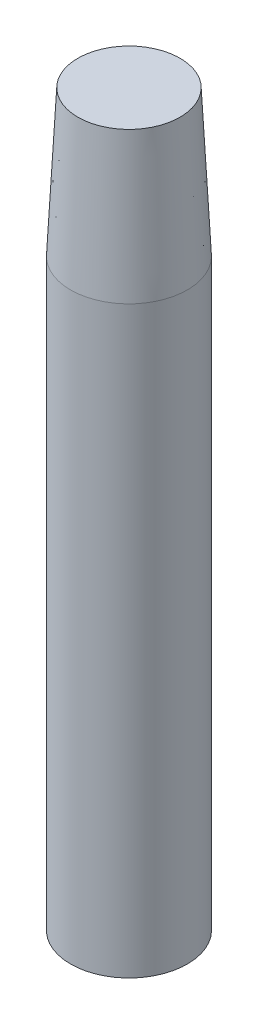
SolidWorks part; units mm, degrees
ref_plane "Front Plane" through (0, 0, 0) normal (0, 0, 1) x (1, 0, 0)
ref_plane "Top Plane" through (0, 0, 0) normal (0, 1, 0) x (1, 0, 0)
ref_plane "Right Plane" through (0, 0, 0) normal (1, 0, 0) x (0, 0, -1)
sketch "Sketch1" plane through (0, 0, 0) normal (0, 1, 0) x (1, 0, 0)
  circle A0 centre (0, 0) radius 4
  dimension "D1" = 8
extrude "Boss-Extrude1" add sketch "Sketch1" along normal blind 50
chamfer "Chamfer1" distance 10 distance2 0.5 1 edges at (0, 50, 4)
hole_wizard "M4 Tapped Hole1" positions "Sketch4" profile "Sketch3" tap size "M4" standard "Gb"
sketch "Sketch4" plane through (0, 0, 0) normal (0, -1, 0) x (-1, 0, 0)
  point P0 (0, 0)
sketch "Sketch3" plane through (0, 0, 0) normal (1, 0, 0) x (0, 0, -1)
  line L0 (0, 0) -> (0, 11.0914)
  line L1 (0, 11.0914) -> (1.65, 10.1)
  line L2 (1.65, 10.1) -> (1.65, 0)
  line L5 (1.65, 0) -> (0, 0)
  line L10 (0, 11.0914) -> (-1.65, 10.1) construction
  line L11 (0, -6.35) -> (0, 107.95) construction
  dimension "螺纹孔钻头直径" = 3.3
  dimension "螺纹孔钻头深度" = 10.1
  dimension "导头角度" = 118
cosmetic thread "Hole Thread 1"
